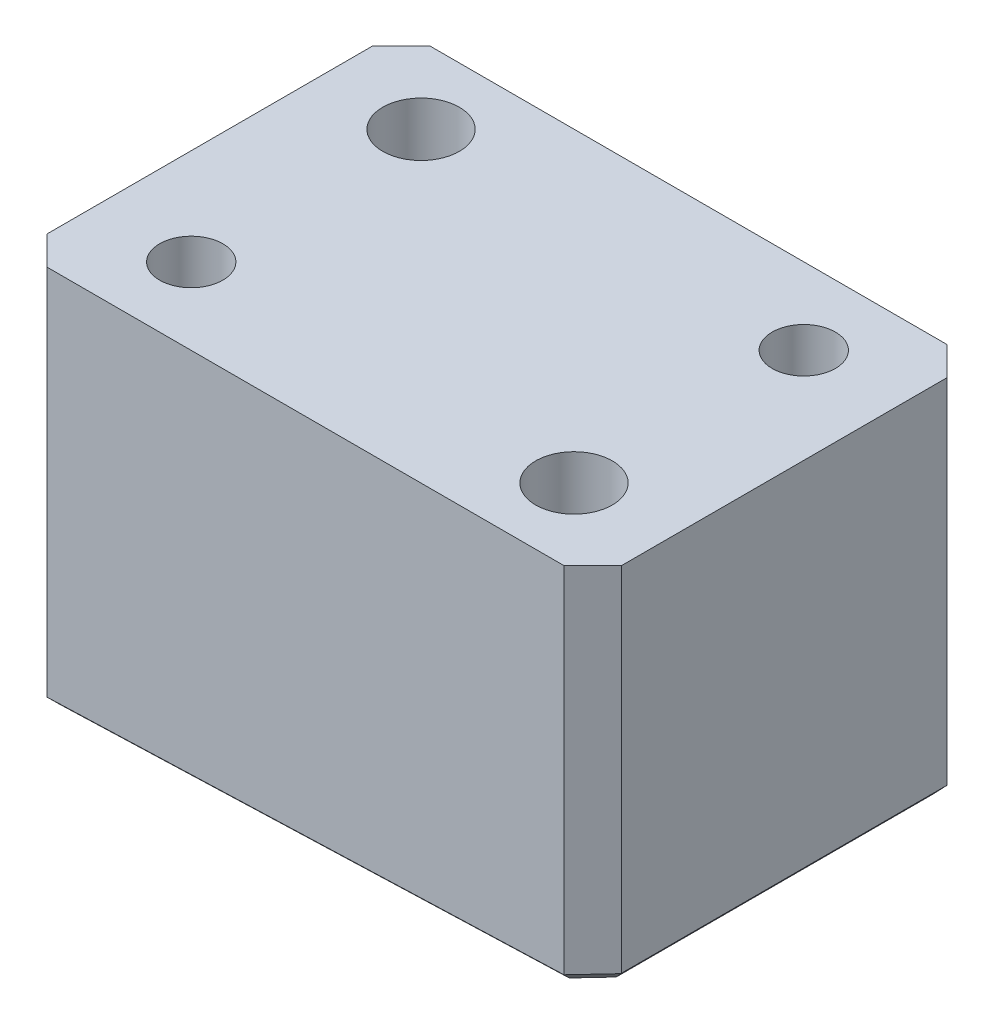
from build123d import *
from OCP.BRepFilletAPI import BRepFilletAPI_MakeChamfer

# Parameters (mm, degrees)
BOSS_EXTRUDE1_DEPTH        = 40
CHAMFER1_SIZE              = 3
CHAMFER2_SIZE              = 1
CHAMFER2_SIZE2             = 0.96684652
CHAMFER2_SIZE2_2           = 1.036815955
CHAMFER2_SIZE2_3           = 0.976206784
CHAMFER2_SIZE2_4           = 1.025622313
HOLE2_D                    = 6.6
HOLE2_DEPTH                = 20
SKETCH11_W                 = 5.5
SKETCH11_H                 = 19.966257543
HOLE3_AT_2_COUNT           = 2
HOLE3_AT_2_PITCH           = 46.626722383
SIZE_MM_BLIND_HOLE_1_D     = 8
SIZE_MM_BLIND_HOLE_1_DEPTH = 12.5
SIZE_MM_BLIND_HOLE_1_TIP   = 2.403442476


with BuildPart() as part:
    # Sketch2 → Boss-Extrude1 (new body)
    with BuildSketch(Plane.XY):
        Polygon((-37.58146769, 20.630053858), (22.41853231, 22.725300027), (22.41853231, 60.630053858), (-37.58146769, 60.630053858), align=None)
    extrude(amount=BOSS_EXTRUDE1_DEPTH)

    # Chamfer1
    chamfer1_edges = [part.edges().sort_by_distance(p)[0] for p in [
        (22.41853231, 41.677676942, 40),
        (-37.58146769, 40.630053858, 40),
        (22.41853231, 41.677676942, 0),
        (-37.58146769, 40.630053858, 0),
    ]]
    chamfer(chamfer1_edges, length=CHAMFER1_SIZE)

    # Chamfer2: one chamfer whose edges measure the first distance from different faces: ONE call of the kernel's chamfer builder (chamfer() names one face for all edges)
    chamfer2_edges_1 = [part.edges().sort_by_distance(p)[0] for p in [
        (-37.58146769, 20.630053858, 20),
    ]]
    chamfer2_side_1 = [part.faces().sort_by_distance(p)[0] for p in [
        (-37.58146769, 40.630053858, 20),
    ]]
    chamfer2_edges_2 = [part.edges().sort_by_distance(p)[0] for p in [
        (-7.58146769, 21.677676942, 0),
        (-7.58146769, 21.677676942, 40),
    ]]
    chamfer2_edges_3 = [part.edges().sort_by_distance(p)[0] for p in [
        (22.41853231, 22.725300027, 20),
    ]]
    chamfer2_side_3 = [part.faces().sort_by_distance(p)[0] for p in [
        (-7.58146769, 21.677676942, 20),
    ]]
    chamfer2_edges_4 = [part.edges().sort_by_distance(p)[0] for p in [
        (-36.08146769, 20.682435012, 38.5),
    ]]
    chamfer2_side_4 = [part.faces().sort_by_distance(p)[0] for p in [
        (-36.082123313, 40.656232987, 38.499344377),
    ]]
    chamfer2_edges_5 = [part.edges().sort_by_distance(p)[0] for p in [
        (20.91853231, 22.672918873, 38.5),
    ]]
    chamfer2_side_5 = [part.faces().sort_by_distance(p)[0] for p in [
        (20.917842306, 41.651474317, 38.500690004),
    ]]
    chamfer2_edges_6 = [part.edges().sort_by_distance(p)[0] for p in [
        (20.91853231, 22.672918873, 1.5),
    ]]
    chamfer2_side_6 = [part.faces().sort_by_distance(p)[0] for p in [
        (20.917842306, 41.651474317, 1.499309996),
    ]]
    chamfer2_edges_7 = [part.edges().sort_by_distance(p)[0] for p in [
        (-36.08146769, 20.682435012, 1.5),
    ]]
    chamfer2_side_7 = [part.faces().sort_by_distance(p)[0] for p in [
        (-36.082123313, 40.656232987, 1.500655623),
    ]]
    chamfer2 = BRepFilletAPI_MakeChamfer(part.part.solid().wrapped)
    for e in chamfer2_edges_1:
        chamfer2.Add(CHAMFER2_SIZE, CHAMFER2_SIZE2, e.wrapped, chamfer2_side_1[0].wrapped)  # the first distance lies on this face
    for e in chamfer2_edges_2:
        chamfer2.Add(CHAMFER2_SIZE, e.wrapped)
    for e in chamfer2_edges_3:
        chamfer2.Add(CHAMFER2_SIZE, CHAMFER2_SIZE2_2, e.wrapped, chamfer2_side_3[0].wrapped)  # the first distance lies on this face
    for e in chamfer2_edges_4:
        chamfer2.Add(CHAMFER2_SIZE, CHAMFER2_SIZE2_3, e.wrapped, chamfer2_side_4[0].wrapped)  # the first distance lies on this face
    for e in chamfer2_edges_5:
        chamfer2.Add(CHAMFER2_SIZE, CHAMFER2_SIZE2_4, e.wrapped, chamfer2_side_5[0].wrapped)  # the first distance lies on this face
    for e in chamfer2_edges_6:
        chamfer2.Add(CHAMFER2_SIZE, CHAMFER2_SIZE2_4, e.wrapped, chamfer2_side_6[0].wrapped)  # the first distance lies on this face
    for e in chamfer2_edges_7:
        chamfer2.Add(CHAMFER2_SIZE, CHAMFER2_SIZE2_3, e.wrapped, chamfer2_side_7[0].wrapped)  # the first distance lies on this face
    add(Compound.cast(chamfer2.Shape()), mode=Mode.REPLACE)

    # Hole2
    with Locations(Plane(origin=(0, 60.630053858, 0), x_dir=(1, 0, 0), z_dir=(0, 1, 0))):
        with Locations((-27.514846728, -32), (12.460786352, -8)):
            Hole(HOLE2_D / 2, depth=HOLE2_DEPTH)

    # Sketch11 → Hole3 (revolve, cut)
    with BuildSketch(Plane(origin=(-27.514846728, 40.630053858, 32), x_dir=(0, 0, 1), z_dir=(1, 0, 0))):
        with Locations((2.75, 9.983128772)):
            Rectangle(SKETCH11_W, SKETCH11_H)
    hole3 = revolve(axis=Axis((-27.514846728, -69.369946142, 32), (0, 1, 0)), mode=Mode.SUBTRACT)

    # Hole3 at 2: Hole3 ×2
    with Locations(*[Vector(0.8573545605919571, 0, -0.514726293705861) * (i * HOLE3_AT_2_PITCH) for i in range(1, HOLE3_AT_2_COUNT)]):
        add(hole3, mode=Mode.SUBTRACT)

    # Size mm blind hole 1
    with Locations(Plane(origin=(0, 60.630053858, 0), x_dir=(1, 0, 0), z_dir=(0, 1, 0))):
        with Locations((-27.514846728, -8), (12.460786352, -32)):
            Hole(SIZE_MM_BLIND_HOLE_1_D / 2, depth=SIZE_MM_BLIND_HOLE_1_DEPTH)
            with Locations((0, 0, -(SIZE_MM_BLIND_HOLE_1_DEPTH + SIZE_MM_BLIND_HOLE_1_TIP / 2))):  # 118° drill point
                Cone(0, SIZE_MM_BLIND_HOLE_1_D / 2, SIZE_MM_BLIND_HOLE_1_TIP, mode=Mode.SUBTRACT)


solid = part.part
